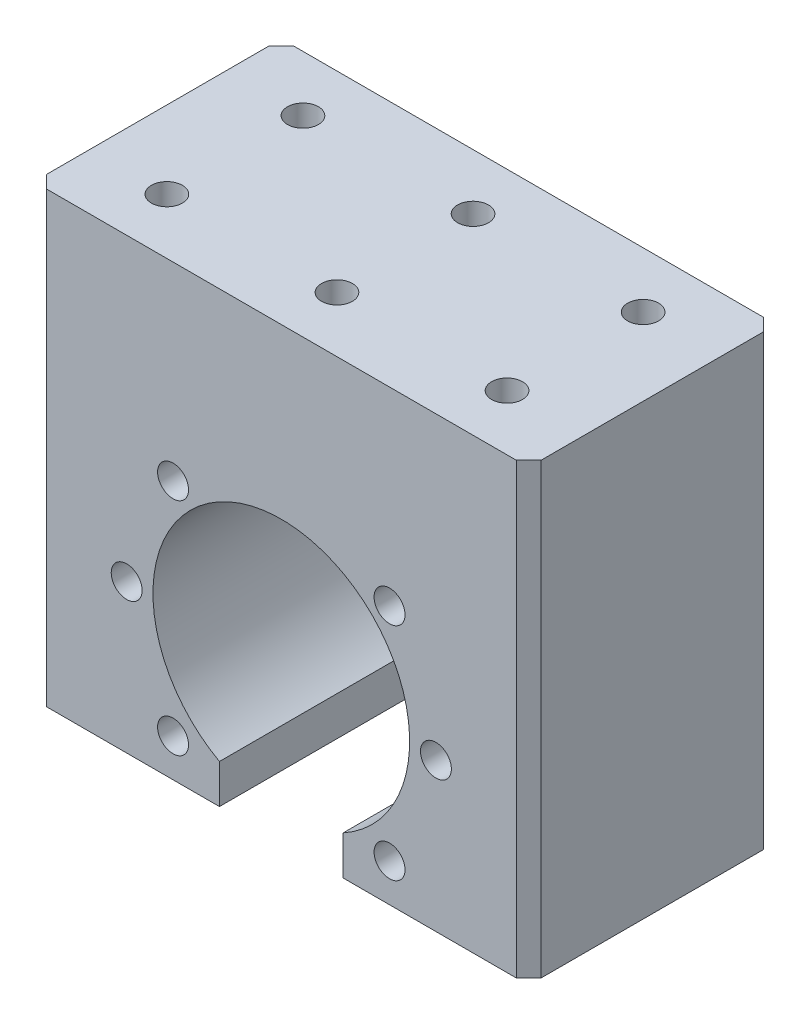
from build123d import *

# Parameters (mm, degrees)
SKETCH_1_W             = 80
SKETCH_1_H             = 72.5
SKETCH_1_R             = 20.75
EXTRUDE_1_DEPTH        = 20
SKETCH_2_W             = 20
SKETCH_2_H             = 6.318622164
CUT_EXTRUDE_1_DEPTH    = 68.186773252
HOLE_WIZARD_M6_1_D     = 5
HOLE_WIZARD_M6_2_D     = 5
HOLE_WIZARD_M6_2_DEPTH = 15
HOLE_WIZARD_M6_2_TIP   = 1.502151548
CHAMFER_1_SIZE         = 2


with BuildPart() as part:
    # 草图1 → 凸台-拉伸1 (new, symmetric)
    with BuildSketch(Plane.XY):
        Rectangle(SKETCH_1_W, SKETCH_1_H)
        with Locations((0, -11.75)):
            Circle(SKETCH_1_R, mode=Mode.SUBTRACT)
    extrude(amount=EXTRUDE_1_DEPTH, both=True)

    # 草图2 → 切除-拉伸1 (cut, through all)
    with BuildSketch(Plane.XY.offset(20)):
        with Locations((0, -33.090688918)):
            Rectangle(SKETCH_2_W, SKETCH_2_H)
    extrude(amount=-CUT_EXTRUDE_1_DEPTH, mode=Mode.SUBTRACT)

    # M6 螺纹孔1 (through all)
    with Locations(Plane(origin=(0, 0, -20), x_dir=(-1, 0, 0), z_dir=(0, 0, -1))):
        with Locations((-17.5, 5.603571071), (17.5, 5.603571071), (17.5, -30.103571071), (-17.5, -30.103571071), (-25, -12.25), (25, -12.25)):
            Hole(HOLE_WIZARD_M6_1_D / 2)

    # M6 螺纹孔2
    with Locations(Plane(origin=(0, 36.25, 0), x_dir=(1, 0, 0), z_dir=(0, 1, 0))):
        with Locations((-27.5, 11), (-27.5, -11), (27.5, -11), (27.5, 11), (0, 11), (0, -11)):
            Hole(HOLE_WIZARD_M6_2_D / 2, depth=HOLE_WIZARD_M6_2_DEPTH)
            with Locations((0, 0, -(HOLE_WIZARD_M6_2_DEPTH + HOLE_WIZARD_M6_2_TIP / 2))):  # 118° drill point
                Cone(0, HOLE_WIZARD_M6_2_D / 2, HOLE_WIZARD_M6_2_TIP, mode=Mode.SUBTRACT)

    # 倒角1
    chamfer_1_edges = [part.edges().sort_by_distance(p)[0] for p in [
        (-40, 0, 20),
        (40, 0, 20),
        (-40, 0, -20),
        (40, 0, -20),
    ]]
    chamfer(chamfer_1_edges, length=CHAMFER_1_SIZE)


solid = part.part
